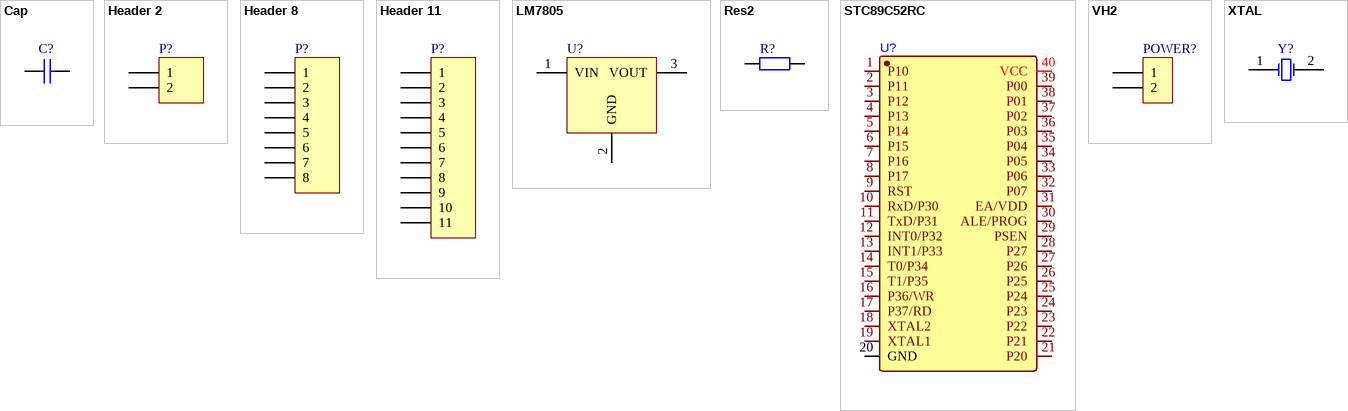
[diagram p0: symbols Cap to XTAL]
# Altium schematic symbol library MISC82800-3.SCHLIB: 9 symbols
Pins are listed as number, name and electrical type; pins without a type are passive.


## Cap
designator C?
Capacitor
footprint RAD-0.3 (Radial Cap, Thru-Hole; 2 Leads; 0.3 in Pin Spacing)
simulation model CAP (Capacitor)
signal-integrity model Cap
pins: 1, 2

## Header 2
designator P?
Header, 2-Pin
footprint HDR1X2 (Connector; Header; 2 Position)
signal-integrity model Connector
pins: 1, 2

## Header 8
designator P?
Header, 8-Pin
footprint HDR1X8 (Connector; Header; 8 Position)
signal-integrity model Connector
pins: 1, 2, 3, 4, 5, 6, 7, 8

## Header 11
designator P?
Header, 11-Pin
footprint HDR1X11 (Connector; Header; 11 Position)
signal-integrity model Connector
pins: 1, 2, 3, 4, 5, 6, 7, 8, 9, 10, 11

## LM7805
designator U?
footprint TO220A (220, 3-pin transistor)
footprint TO252 (252 transistor)
pins: 1 VIN, 2 GND, 3 VOUT

## Res2
designator R?
Resistor
footprint AXIAL-0.4 (Axial Device, Thru-Hole; 2 Leads; 0.4 in Pin Spacing)
simulation model RESISTOR (Resistor)
signal-integrity model Res
pins: 1, 2

## STC89C52RC
designator U?
footprint STC89C52RC
pins: 1 P10, 2 P11, 3 P12, 4 P13, 5 P14, 6 P15, 7 P16, 8 P17, 9 RST, 10 RxD/P30, 11 TxD/P31, 12 INT0/P32, 13 INT1/P33, 14 T0/P34, 15 T1/P35, 16 P36/WR, 17 P37/RD, 18 XTAL2, 19 XTAL1, 20 GND, 21 P20, 22 P21, 23 P22, 24 P23, 25 P24, 26 P25, 27 P26, 28 P27, 29 PSEN, 30 ALE/PROG, 31 EA/VDD, 32 P07, 33 P06, 34 P05, 35 P04, 36 P03, 37 P02, 38 P01, 39 P00, 40 VCC

## VH2
designator POWER?
footprint VH3.96-2A
footprint VH3.96-2AW
footprint VH3.96-2AWD
pins: 1, 2

## XTAL
designator Y?
Crystal Oscillator
footprint R38 (Crystal, Thru-Hole; 2 Leads; Body 3.1 x 8.2 mm (Dia.xH))
simulation model XTAL (Spice Subcircuit)
pins: 1 OSC1, 2 OSC2